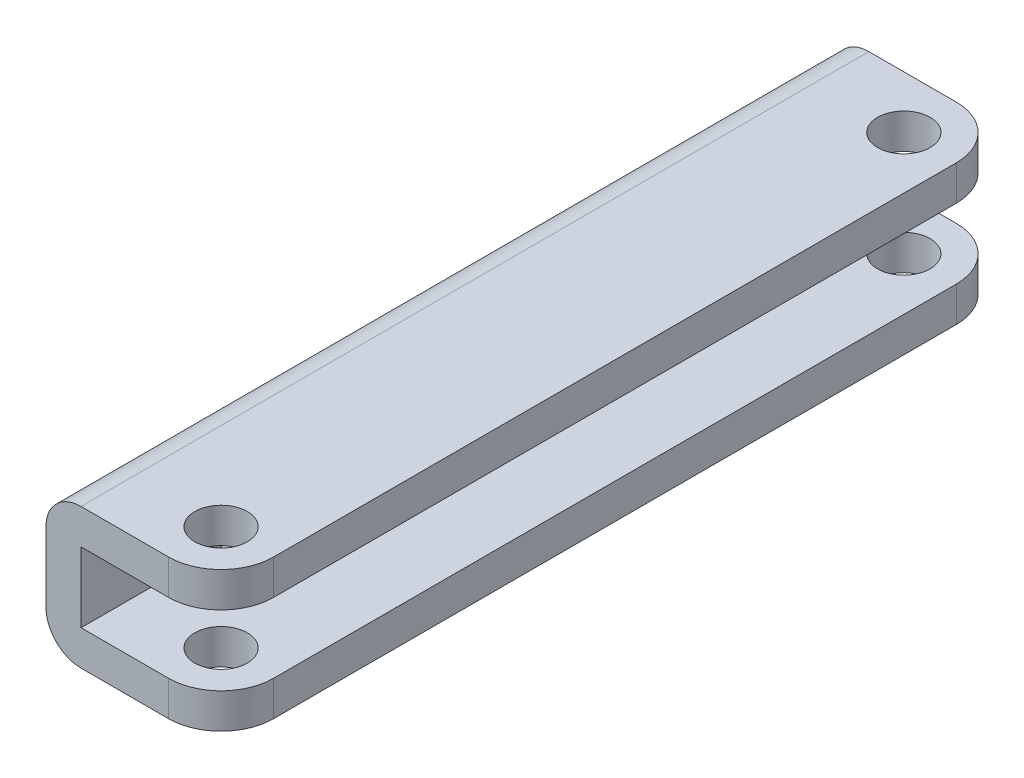
from build123d import *

# Parameters (mm, degrees)
BOSS_EXTRUDE1_DEPTH = 45
SKETCH2_R           = 1.5
CUT_EXTRUDE1_DEPTH  = 47.786750261
FILLET1_R           = 3


with BuildPart() as part:
    # Sketch1 → Boss-Extrude1 (new body)
    with BuildSketch(Plane.XY):
        with BuildLine():
            Line((0, 4), (0, 2))
            Line((0, 2), (-8, 2))
            Line((-8, 2), (-8, -2))
            Line((-8, -2), (0, -2))
            Line((0, -2), (0, -4))
            Line((0, -4), (-8, -4))
            ThreePointArc((-8, -4), (-9.414213562, -3.414213562), (-10, -2))
            Line((-10, -2), (-10, 2))
            ThreePointArc((-10, 2), (-9.414213562, 3.414213562), (-8, 4))
            Line((-8, 4), (0, 4))
        make_face()
    extrude(amount=BOSS_EXTRUDE1_DEPTH)

    # Sketch2 → Cut-Extrude1 (cut, through all)
    with BuildSketch(Plane(origin=(0, -4, 0), x_dir=(-1, 0, 0), z_dir=(0, -1, 0))):
        with Locations(Location((3, -3, 0), (0, 0, 180))):
            Circle(SKETCH2_R)
        with Locations(Location((3, -42, 0), (0, 0, 180))):
            Circle(SKETCH2_R)
    extrude(amount=-CUT_EXTRUDE1_DEPTH, mode=Mode.SUBTRACT)

    # Fillet1
    fillet1_edges = [part.edges().sort_by_distance(p)[0] for p in [
        (0, 3, 0),
        (0, -3, 0),
        (0, 3, 45),
        (0, -3, 45),
    ]]
    fillet(fillet1_edges, radius=FILLET1_R)


solid = part.part
